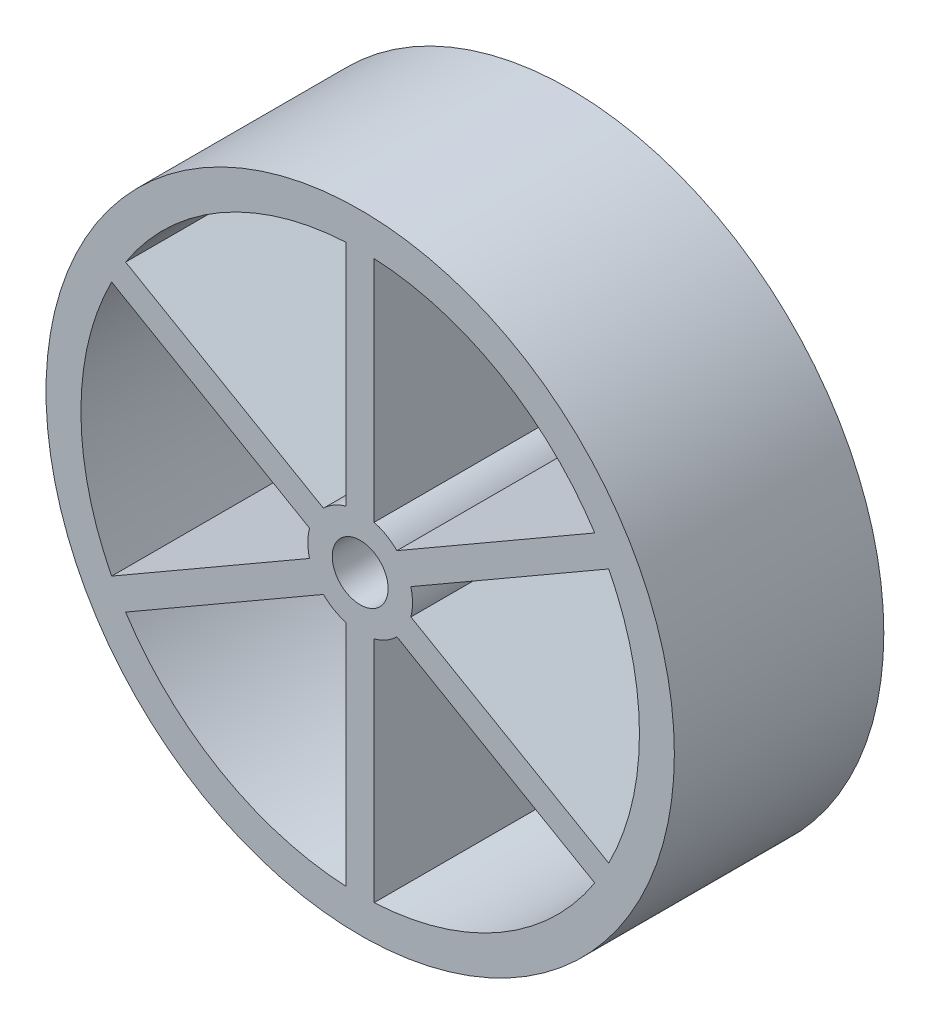
SolidWorks part; units mm, degrees
ref_plane "Front Plane" through (0, 0, 0) normal (0, 0, 1) x (1, 0, 0)
ref_plane "Top Plane" through (0, 0, 0) normal (0, 1, 0) x (1, 0, 0)
ref_plane "Right Plane" through (0, 0, 0) normal (1, 0, 0) x (0, 0, -1)
other "Configuration Table"
sketch "Sketch1" plane through (0, 0, 0) normal (0, 0, 1) x (1, 0, 0)
  circle A0 centre (10, -61.7532) radius 7.5
  dimension "D1" = 15
extrude "Boss-Extrude1" add sketch "Sketch1" along normal blind 30
sketch "Sketch2" plane through (0, 0, 30) normal (0, 0, 1) x (1, 0, 0)
  circle A0 centre (10, -61.7532) radius 40
  dimension "D1" = 80
extrude "Extrude-Thin1" add sketch "Sketch2" against normal blind 30 separate body thin
sketch "Sketch5" plane through (0, 0, 30) normal (0, 0, 1) x (1, 0, 0)
  line L0 (10, -57.4586) -> (10, -21.1294)
extrude "Extrude-Thin3" add sketch "Sketch5" against normal blind 30 thin thin type mid plane wall 4
pattern_circular "CirPattern4" count 6 over 360 about axis through (10, -61.7532, 0) along (0, 0, 1) of "Extrude-Thin3"
sketch "Sketch6" plane through (0, 0, 30) normal (0, 0, 1) x (1, 0, 0)
  circle A0 centre (10, -61.7532) radius 4
  dimension "D1" = 8
extrude "Cut-Extrude1" cut sketch "Sketch6" against normal through all both and the other way through all
